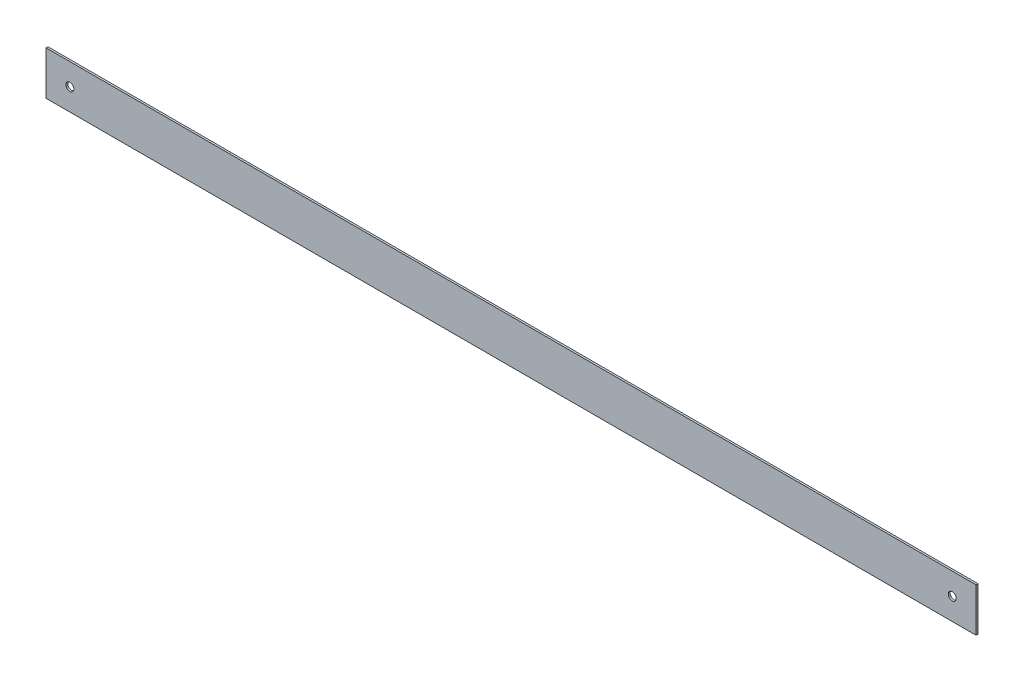
from build123d import *

# Parameters (mm, degrees)
SKETCH_1_W                = 585
SKETCH_1_H                = 27.5
EXTRUDE_1_DEPTH           = 1.2
HOLE_WIZARD_5_0_5_1_D     = 5
HOLE_WIZARD_5_0_5_1_DEPTH = 5
HOLE_WIZARD_5_0_5_1_TIP   = 1.502151548


with BuildPart() as part:
    # 草图1 → 凸台-拉伸1 (new body)
    with BuildSketch(Plane.XY):
        with Locations((292.5, 13.75)):
            Rectangle(SKETCH_1_W, SKETCH_1_H)
    extrude(amount=EXTRUDE_1_DEPTH)

    # Ø5.0 (5) 直径孔1
    with Locations(Plane.XY.offset(1.2)):
        with Locations((15, 13.75), (570, 13.75)):
            Hole(HOLE_WIZARD_5_0_5_1_D / 2, depth=HOLE_WIZARD_5_0_5_1_DEPTH)
            with Locations((0, 0, -(HOLE_WIZARD_5_0_5_1_DEPTH + HOLE_WIZARD_5_0_5_1_TIP / 2))):  # 118° drill point
                Cone(0, HOLE_WIZARD_5_0_5_1_D / 2, HOLE_WIZARD_5_0_5_1_TIP, mode=Mode.SUBTRACT)


solid = part.part
